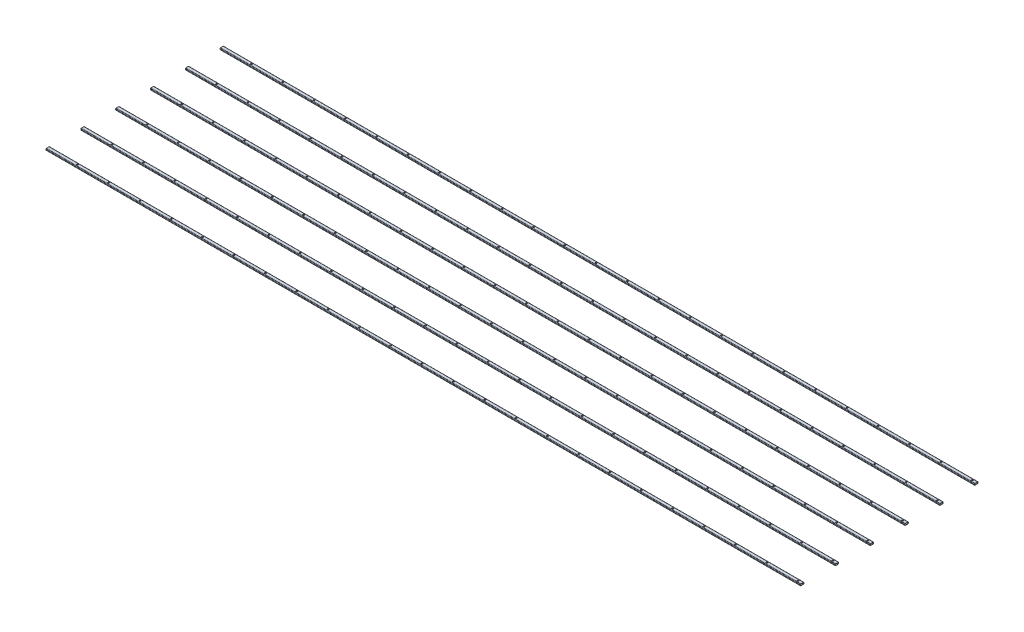
SolidWorks part; units mm, degrees
material "AISI 304"
ref_plane "Front Plane" through (0, 0, 0) normal (0, 0, 1) x (1, 0, 0)
ref_plane "Top Plane" through (0, 0, 0) normal (0, 1, 0) x (1, 0, 0)
ref_plane "Right Plane" through (0, 0, 0) normal (1, 0, 0) x (0, 0, -1)
sketch3d "3DSketch1"
  line L0 (0, 0, 0) -> (0, 0, -1500)
  line L1 (0, 0, -1500) -> (6500, 0, -1500)
  line L2 (6500, 0, -1500) -> (6500, 0, 0)
  line L3 (0, 0, 0) -> (6500, 0, 0)
  line L4 (0, 0, -1200) -> (6500, 0, -1200)
  line L5 (0, 0, -900) -> (6500, 0, -900)
  line L6 (0, 0, -600) -> (6500, 0, -600)
  line L7 (0, 0, -300) -> (6500, 0, -300)
  line L8 (0, 0, 0) -> (0, 0, 300) construction
  line L9 (0, 0, 300) -> (5200, 0, 300)
  dimension "D1" = 6500
  dimension "D2" = 1500
  dimension "D3" = 1500
  dimension "D4" = 300
  dimension "D5" = 600
  dimension "D6" = 300
  dimension "D7" = 300
  dimension "D8" = 300
  dimension "D9" = 5200
other "Gb/6728-1986 rectangular hollow section 030 X 20 X 2"
ref_plane "Plane1" through (0, 0, -1500) normal (1, 0, 0) x (0, -1, 0)
sketch "Sketch17" plane through (0, 0, -1500) normal (1, 0, 0) x (0, -1, 0)
  line L0 (-3.5, -13) -> (3.5, -13)
  line L1 (-5.5, -11) -> (-5.5, 11)
  line L2 (3.5, 13) -> (-3.5, 13)
  line L3 (5.5, 11) -> (5.5, -11)
  line L4 (-3.5, -15) -> (3.5, -15)
  line L5 (-7.5, -11) -> (-7.5, 11)
  line L6 (3.5, 15) -> (-3.5, 15)
  line L7 (7.5, 11) -> (7.5, -11)
  arc A0 (7.5, 11) -> (3.5, 15) centre (3.5, 11) ccw
  arc A1 (3.5, -15) -> (7.5, -11) centre (3.5, -11) ccw
  arc A2 (-7.5, -11) -> (-3.5, -15) centre (-3.5, -11) ccw
  arc A3 (-3.5, 15) -> (-7.5, 11) centre (-3.5, 11) ccw
  arc A4 (-3.5, 13) -> (-5.5, 11) centre (-3.5, 11) ccw
  arc A5 (5.5, 11) -> (3.5, 13) centre (3.5, 11) ccw
  arc A6 (3.5, -13) -> (5.5, -11) centre (3.5, -11) ccw
  arc A7 (-5.5, -11) -> (-3.5, -13) centre (-3.5, -11) ccw
  point P0 (0, 15)
  point P1 (7.5, 0)
  point P2 (0, -15)
  point P3 (-7.5, 0)
  point P4 (-7.5, 15)
  point P5 (7.5, 15)
  point P6 (7.5, -15)
  point P7 (-7.5, -15)
  point P8 (0, 0)
  point P33 (0, 0)
  dimension "D1" = 4
  dimension "Thickness" = 2
  dimension "V_leg" = 30
  dimension "H_leg" = 15
sketch "Sketch4" plane through (0, 7.5, 0) normal (0, 1, 0) x (1, 0, 0)
  line L0 (5200, 1350) -> (4999.3572, 1350) construction
  line L2 (4063, 1548.3609) -> (4160, 1350)
  line L3 (3956.6562, 1496.358) -> (3956.6562, 1377.9802) construction
  line L4 (4063, 1389) -> (4063, 1324) construction
  arc A0 (4063, 1548.3609) -> (3956.6562, 1377.9802) centre (3956.6562, 1496.358) ccw
sketch "Sketch6" plane through (0, 7.5, 0) normal (0, 1, 0) x (1, 0, 0)
  line L0 (0, 1500) -> (6500, 1500) construction
  line L1 (6500, 1500) -> (0, 1500) construction
  line L2 (6500, 1511) -> (6500, 1489) construction
  circle A0 centre (6465, 1500) radius 6.5
  dimension "D2" = 13
  dimension "D1" = 35
extrude "Cut-Extrude1" cut sketch "Sketch6" against normal through all
pattern_linear "LPattern2" count 6 spacing 300 along (0, 0, 1) count 24 spacing 270 along (-1, 0, 0) of "Cut-Extrude1"
